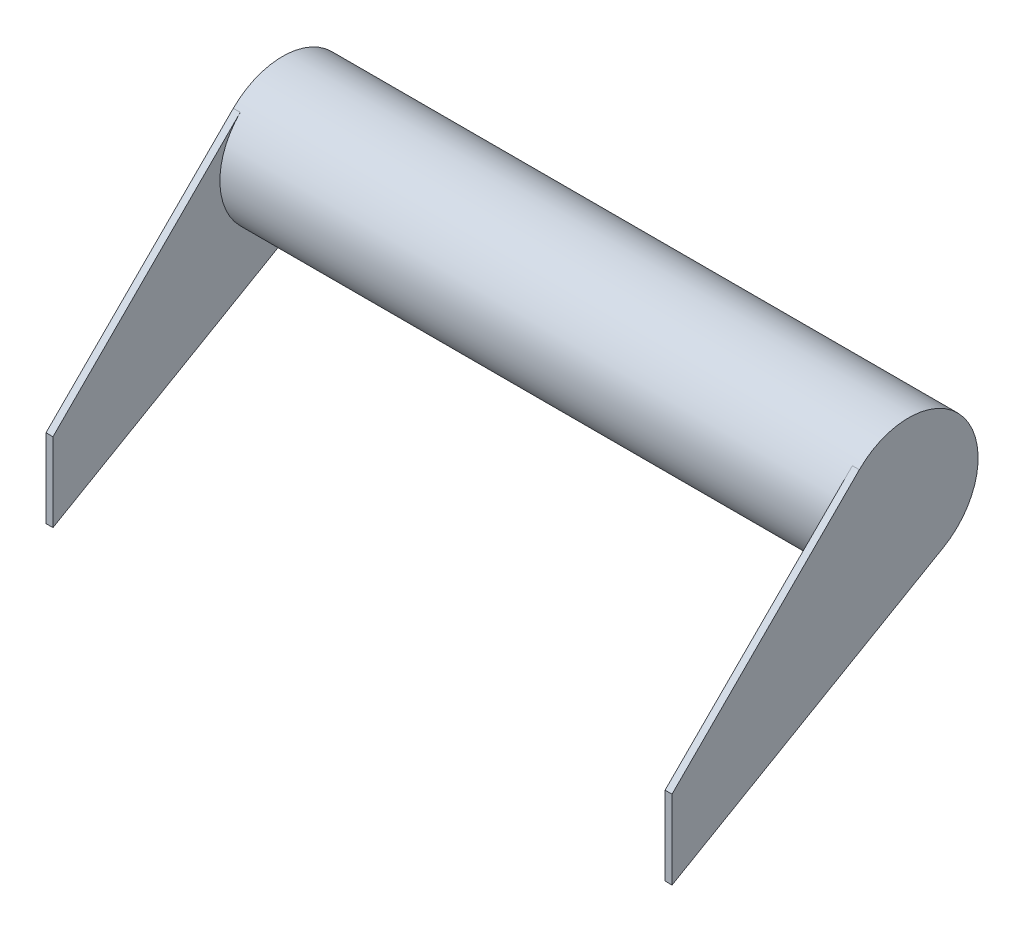
SolidWorks part; units mm, degrees
material "AISI 304"
ref_plane "Front Plane" through (0, 0, 0) normal (0, 0, 1) x (1, 0, 0)
ref_plane "Top Plane" through (0, 0, 0) normal (0, 1, 0) x (1, 0, 0)
ref_plane "Right Plane" through (0, 0, 0) normal (1, 0, 0) x (0, 0, -1)
sketch "Sketch1" plane through (0, 0, 0) normal (1, 0, 0) x (0, 0, -1)
  circle A0 centre (0, 0) radius 10
  circle A1 centre (0, 0) radius 9
  dimension "D1" = 20
  dimension "D2" = 1
extrude "Boss-Extrude1" add sketch "Sketch1" along normal mid plane 90
sketch "Sketch2" plane through (45, 0, 0) normal (1, 0, 0) x (0, 0, -1)
  line L0 (-7.0711, 7.0711) -> (-34, -19.8579)
  line L1 (-34, -19.8579) -> (-34, -31.1769)
  line L2 (-34, -31.1769) -> (5, -8.6603)
  line L3 (0, 0) -> (5, -8.6603) construction
  line L4 (0, 0) -> (-7.0711, 7.0711) construction
  line L5 (0, 0) -> (0, 10) construction
  circle A1 centre (0, 0) radius 10
  circle A2 centre (0, 0) radius 10
  circle M6 centre (0, 0) radius 10
  circle M7 centre (0, 0) radius 9
  dimension "D2" = 45
  dimension "D3" = 150
  dimension "D4" = 34
  dimension "D1" = 0
extrude "Boss-Extrude2" add sketch "Sketch2" against normal blind 1 contours L1 L2 L0 M6 | M7 | M6 M7
mirror "Mirror1" about plane through (0, 0, 0) normal (1, 0, 0) of "Boss-Extrude2"
